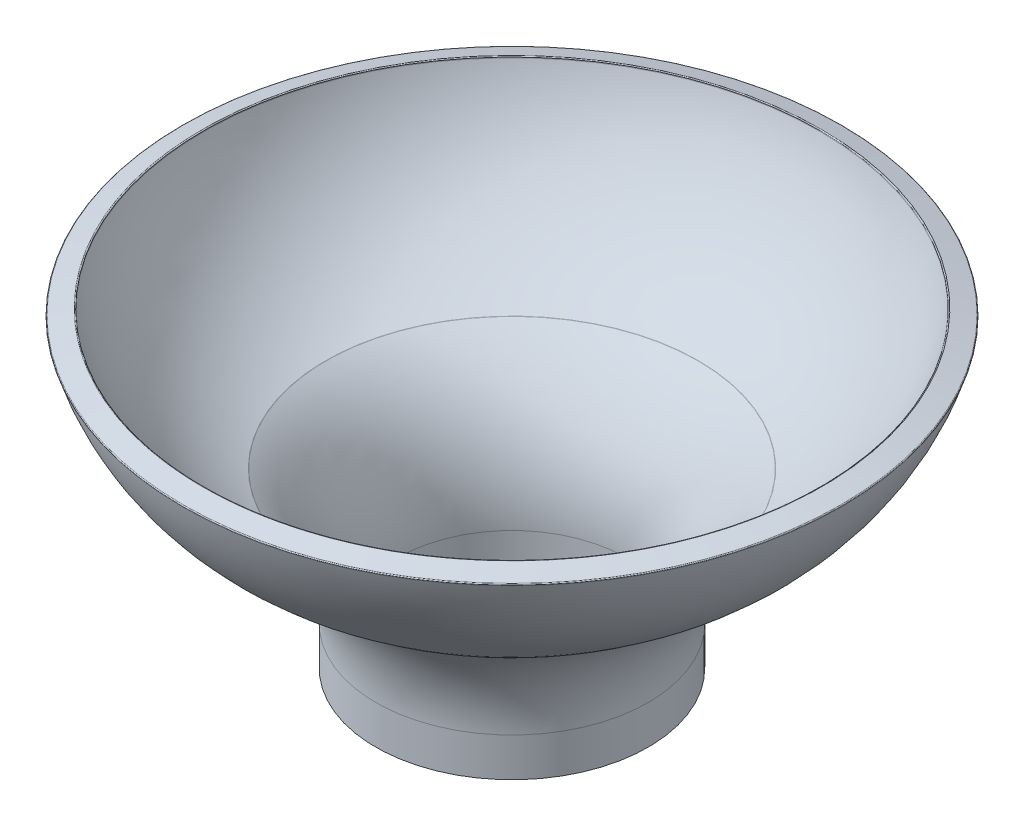
SolidWorks part; units mm, degrees
ref_plane "Front" through (0, 0, 0) normal (0, 0, 1) x (1, 0, 0)
ref_plane "Top" through (0, 0, 0) normal (0, 1, 0) x (1, 0, 0)
ref_plane "Side view" through (0, 0, 0) normal (1, 0, 0) x (0, 0, -1)
sketch "Sketch1" plane through (0, 0, 0) normal (0, 0, 1) x (1, 0, 0)
  line L0 (31.832, -49.6504) -> (31.832, -37.3259)
  line L4 (-29.8944, 49.2954) -> (-29.9524, 49.4868)
  line L5 (24.832, -49.6504) -> (24.832, -37.3259)
  line L6 (-36.5938, 47.266) -> (-36.6517, 47.4574)
  line L7 (24.832, -49.6504) -> (31.832, -49.6504)
  line L8 (-36.4516, 47.8315) -> (-30.3265, 49.6869)
  line L9 (-36.5938, 47.266) -> (-36.7387, 47.7445) construction
  line L10 (-29.8944, 49.2954) -> (-30.0393, 49.7739) construction
  line L11 (68.222, -49.6504) -> (68.222, 62.8412) construction
  arc A0 (8.8702, 5.5335) -> (-29.8944, 49.2954) centre (37.0994, 69.5891) cw
  arc A2 (8.9463, 5.4917) -> (31.832, -37.3259) centre (-19.6653, -37.3259) cw
  arc A6 (8.9463, 5.4917) -> (8.8702, 5.5335) centre (8.6685, 5.076) ccw
  arc A8 (5.5003, -0.6284) -> (24.832, -37.3259) centre (-19.6653, -37.3259) cw
  arc A9 (5.5003, -0.6284) -> (5.5003, -0.6284) centre (5.5003, -0.6284) ccw
  arc A10 (5.5003, -0.6284) -> (-36.5938, 47.266) centre (37.0994, 69.5891) cw
  arc A11 (-36.6517, 47.4574) -> (-36.4516, 47.8315) centre (-36.3646, 47.5444) cw
  arc A12 (-30.3265, 49.6869) -> (-29.9524, 49.4868) centre (-30.2395, 49.3998) cw
  point P19 (8.897, 5.5244)
  dimension "D1" = 7
  dimension "D2" = 0.5
  dimension "D3" = 0.3
  dimension "D4" = 36.39
revolve "Revolution1" add sketch "Sketch1" angle 360 about L11
